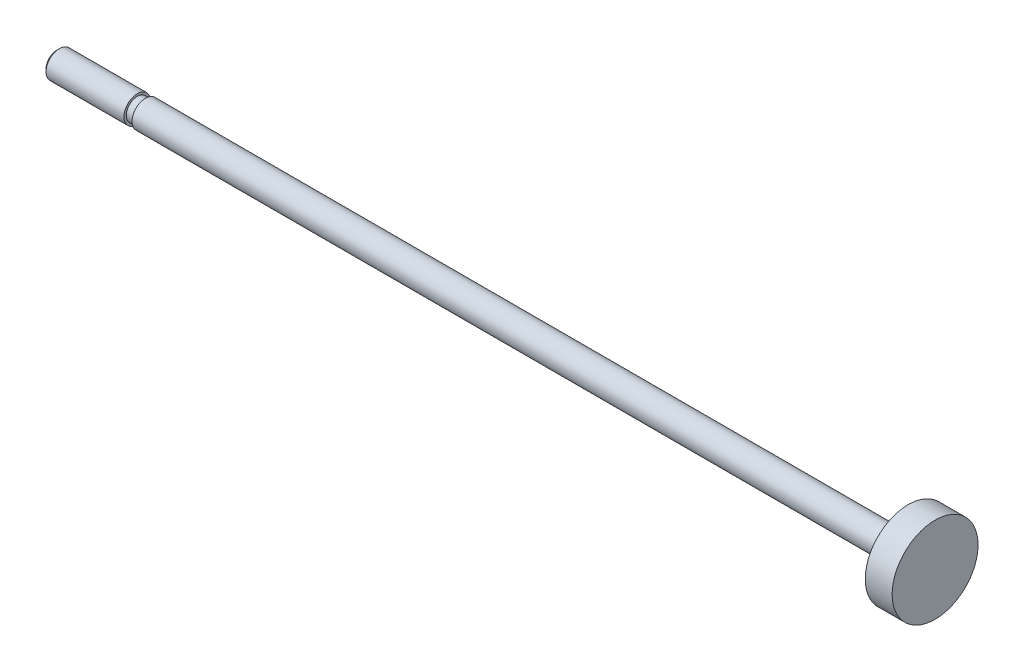
SolidWorks part; units mm, degrees
ref_plane "Front Plane" through (0, 0, 0) normal (0, 0, 1) x (1, 0, 0)
ref_plane "Top Plane" through (0, 0, 0) normal (0, 1, 0) x (1, 0, 0)
ref_plane "Right Plane" through (0, 0, 0) normal (1, 0, 0) x (0, 0, -1)
ref_plane "Plane1" through (0, 0, 0) normal (0, 0, -1) x (-1, 0, 0)
sketch "Sketch1" plane through (0, 0, 0) normal (0, 0, -1) x (-1, 0, 0)
  line L0 (-135.5, 8) -> (-135.5, 0)
  line L1 (-135.5, 0) -> (28, 0)
  line L2 (28, 0) -> (28, 2.0095)
  line L3 (28, 2.0095) -> (27.5095, 2.5)
  line L4 (27.5095, 2.5) -> (13, 2.5)
  line L5 (13, 2.5) -> (13, 2.065)
  line L6 (13, 2.065) -> (11.5, 2.065)
  line L7 (11.5, 2.065) -> (11.5, 2.5)
  line L8 (11.5, 2.5) -> (-130.5, 2.5)
  line L9 (-130.5, 2.5) -> (-130.5, 8)
  line L10 (-130.5, 8) -> (-135.5, 8)
  line L11 (-135.5, 0) -> (28, 0) construction
revolve "Revolve1" add sketch "Sketch1" angle 360 about L11
